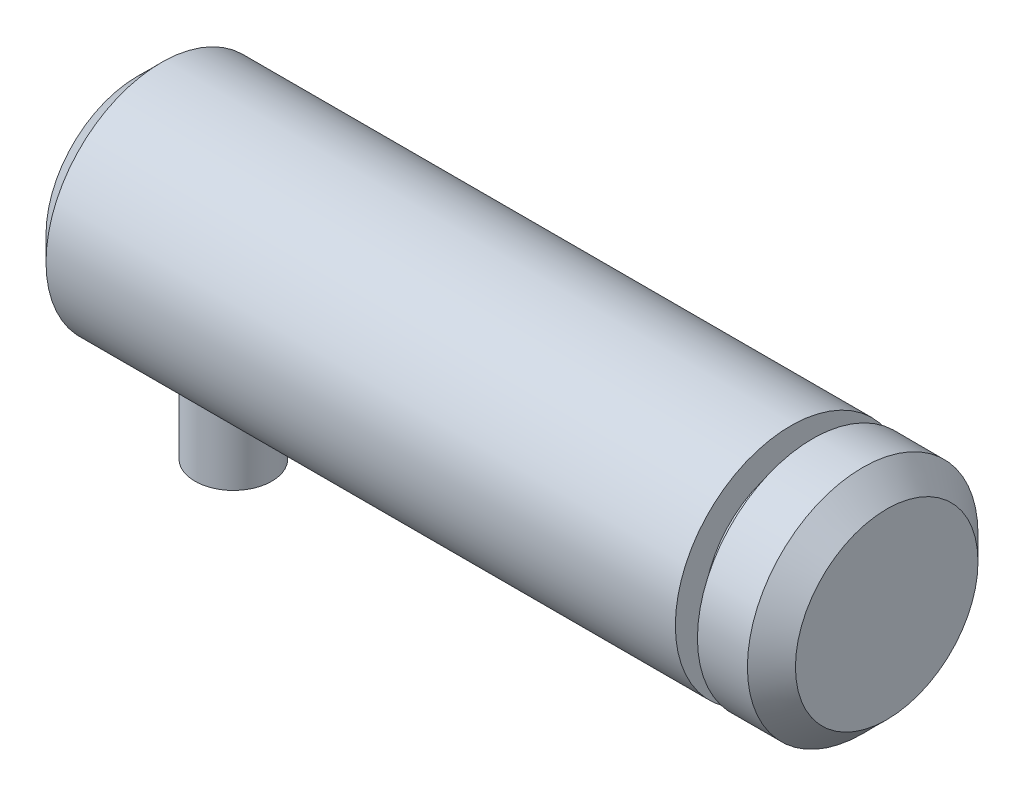
SolidWorks part; units mm, degrees
ref_plane "前视基准面" through (0, 0, 0) normal (0, 0, 1) x (1, 0, 0)
ref_plane "上视基准面" through (0, 0, 0) normal (0, 1, 0) x (1, 0, 0)
ref_plane "右视基准面" through (0, 0, 0) normal (1, 0, 0) x (0, 0, -1)
ref_plane "基准面4" through (0, 0, 0) normal (0, 0, -1) x (-1, 0, 0)
sketch "草图1" plane through (0, 0, 0) normal (0, 0, -1) x (-1, 0, 0)
  line L0 (-19.5, 6) -> (-19.5, 0)
  line L1 (-19.5, 0) -> (19.5, 0)
  line L2 (19.5, 0) -> (19.5, 6)
  line L3 (19.5, 6) -> (-14.5, 6)
  line L4 (-14.5, 6) -> (-14.5, 4.5)
  line L5 (-14.5, 4.5) -> (-15.65, 4.5)
  line L6 (-15.65, 4.5) -> (-15.65, 6)
  line L7 (-15.65, 6) -> (-19.5, 6)
  line L8 (-19.5, 0) -> (19.5, 0) construction
revolve "旋转1" add sketch "草图1" angle 360 about L8
ref_plane "基准面5" through (-14.5, 0, 0) normal (1, 0, 0) x (0, 0, -1)
sketch "草图2" plane through (-14.5, 0, 0) normal (1, 0, 0) x (0, 0, -1)
  line L0 (0, -10) -> (2, -10)
  line L1 (2, -10) -> (2, -5.6569)
  line L2 (2, -5.6569) -> (0, -5.6569)
  line L3 (0, -5.6569) -> (0, -10)
  line L4 (0, -5.6569) -> (0, -10) construction
revolve "旋转2" add sketch "草图2" angle 360 about L4
chamfer "倒角1" distance 1.25 angle 45 2 edges at (-19.5, 0, 6) (19.5, 0, 6)
